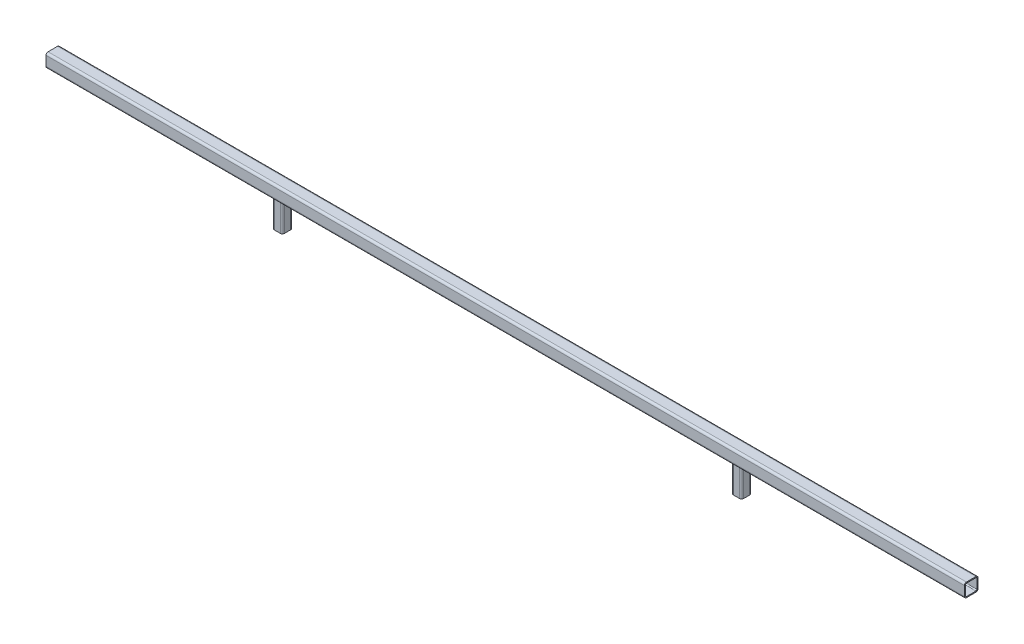
SolidWorks part; units mm, degrees
ref_plane "前视基准面" through (0, 0, 0) normal (0, 0, 1) x (1, 0, 0)
ref_plane "上视基准面" through (0, 0, 0) normal (0, 1, 0) x (1, 0, 0)
ref_plane "右视基准面" through (0, 0, 0) normal (1, 0, 0) x (0, 0, -1)
sketch3d "3D草图1"
  line L0 (-1350, 0, 0) -> (1350, 0, 0)
  line L1 (-675, 0, 0) -> (-675, -100, 0)
  line L2 (675, 0, 0) -> (675, -100, 0)
  point P4 (0, 0, 0)
  dimension "D1" = 2700
  dimension "D2" = 1350
  dimension "D3" = 675
  dimension "D4" = 100
other "冷弯空心方管gb∕t6728-2002 40 X 40 X 3(1)"
ref_plane "基准面1" through (-1350, 0, 0) normal (1, 0, 0) x (0, 0, -1)
sketch "Sketch1" plane through (-1350, 0, 0) normal (1, 0, 0) x (0, 0, -1)
  line L0 (-14, -17) -> (14, -17)
  line L1 (-17, -14) -> (-17, 14)
  line L2 (14, 17) -> (-14, 17)
  line L3 (17, 14) -> (17, -14)
  line L4 (-14, -20) -> (14, -20)
  line L5 (-20, -14) -> (-20, 14)
  line L6 (14, 20) -> (-14, 20)
  line L7 (20, 14) -> (20, -14)
  arc A0 (20, 14) -> (14, 20) centre (14, 14) ccw
  arc A1 (14, -20) -> (20, -14) centre (14, -14) ccw
  arc A2 (-20, -14) -> (-14, -20) centre (-14, -14) ccw
  arc A3 (-14, 20) -> (-20, 14) centre (-14, 14) ccw
  arc A4 (-14, 17) -> (-17, 14) centre (-14, 14) ccw
  arc A5 (17, 14) -> (14, 17) centre (14, 14) ccw
  arc A6 (14, -17) -> (17, -14) centre (14, -14) ccw
  arc A7 (-17, -14) -> (-14, -17) centre (-14, -14) ccw
  point P0 (-20, 0)
  point P1 (20, 0)
  point P2 (0, 20)
  point P3 (0, -20)
  point P4 (0, 0)
  point P5 (-20, -20)
  point P6 (20, -20)
  point P7 (20, 20)
  point P8 (-20, 20)
  point P33 (0, 0)
  dimension "D1" = 6
  dimension "Thickness" = 3
  dimension "V_leg" = 40
other "冷弯空心方管gb∕t6728-2002 30 X 30 X 3(1)"
ref_plane "基准面2" through (-675, 0, 0) normal (0, -1, 0) x (1, 0, 0)
sketch "Sketch11" plane through (-675, 0, 0) normal (0, -1, 0) x (1, 0, 0)
  line L0 (-9, -12) -> (9, -12)
  line L1 (-12, -9) -> (-12, 9)
  line L2 (9, 12) -> (-9, 12)
  line L3 (12, 9) -> (12, -9)
  line L4 (-9, -15) -> (9, -15)
  line L5 (-15, -9) -> (-15, 9)
  line L6 (9, 15) -> (-9, 15)
  line L7 (15, 9) -> (15, -9)
  arc A0 (15, 9) -> (9, 15) centre (9, 9) ccw
  arc A1 (9, -15) -> (15, -9) centre (9, -9) ccw
  arc A2 (-15, -9) -> (-9, -15) centre (-9, -9) ccw
  arc A3 (-9, 15) -> (-15, 9) centre (-9, 9) ccw
  arc A4 (-9, 12) -> (-12, 9) centre (-9, 9) ccw
  arc A5 (12, 9) -> (9, 12) centre (9, 9) ccw
  arc A6 (9, -12) -> (12, -9) centre (9, -9) ccw
  arc A7 (-12, -9) -> (-9, -12) centre (-9, -9) ccw
  point P0 (-15, 0)
  point P1 (15, 0)
  point P2 (0, 15)
  point P3 (0, -15)
  point P4 (0, 0)
  point P5 (-15, -15)
  point P6 (15, -15)
  point P7 (15, 15)
  point P8 (-15, 15)
  point P33 (0, 0)
  dimension "D1" = 6
  dimension "Thickness" = 3
  dimension "V_leg" = 30
other "剪裁/延伸1"
